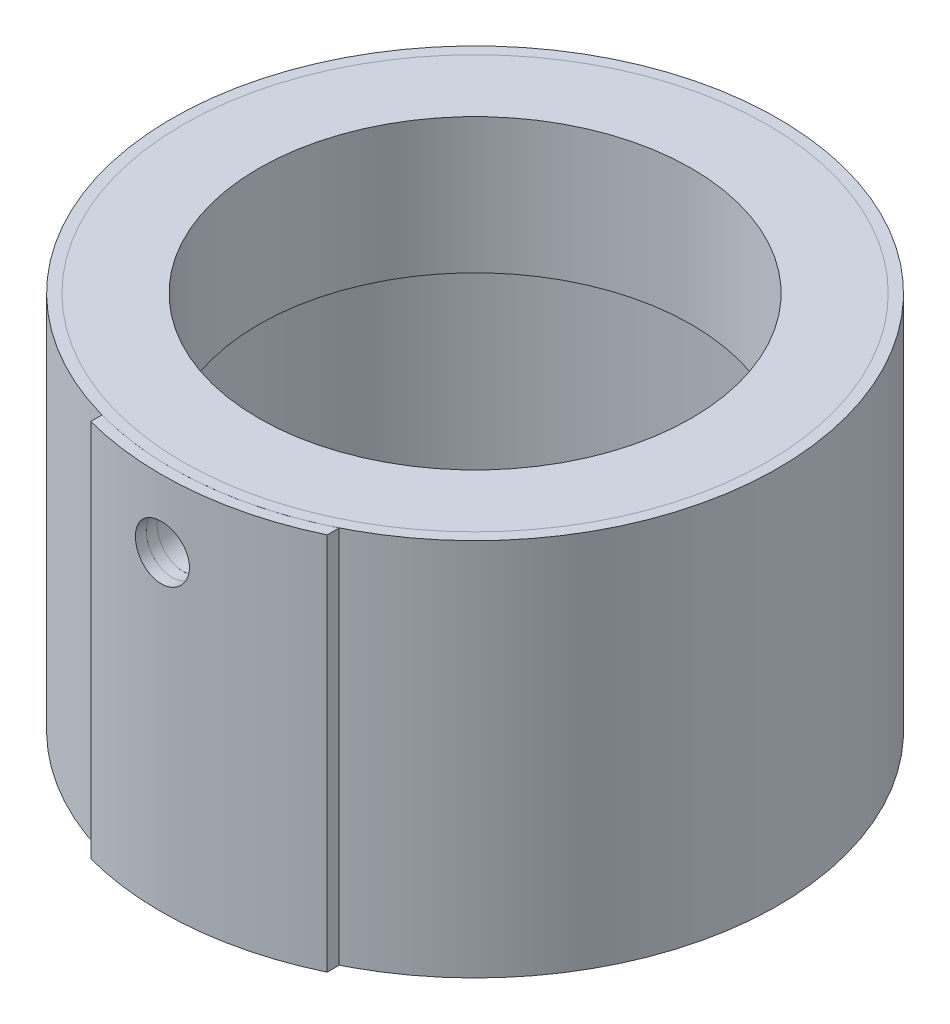
SolidWorks part; units mm, degrees
material "耐油橡胶Ⅰ- 2"
ref_plane "前视基准面" through (0, 0, 0) normal (0, 0, 1) x (1, 0, 0)
ref_plane "上视基准面" through (0, 0, 0) normal (0, 1, 0) x (1, 0, 0)
ref_plane "右视基准面" through (0, 0, 0) normal (1, 0, 0) x (0, 0, -1)
sketch "草图1" plane through (0, 0, 0) normal (0, 1, 0) x (1, 0, 0)
  circle A0 centre (0, 0) radius 40
  circle A1 centre (0, 0) radius 54
  dimension "D1" = 80
  dimension "D2" = 108
extrude "凸台-拉伸1" add sketch "草图1" along normal blind 25
sketch "草图2" plane through (0, 25, 0) normal (0, 1, 0) x (1, 0, 0)
  circle A0 centre (0, 0) radius 54 construction
  circle A1 centre (0, 0) radius 54
  circle A2 centre (0, 0) radius 56
  dimension "D1" = 2
extrude "凸台-拉伸2" add sketch "草图2" against normal blind 70 separate body
sketch "草图4" plane through (0, 25, 0) normal (0, 1, 0) x (1, 0, 0)
  line L0 (0, 0) -> (0, -58) construction
  line L1 (25, -50.1099) -> (25, -52.3355)
  line L2 (-15, -53.9537) -> (-15, -56.0268)
  line L3 (25, 0) -> (25, -58) construction
  line L4 (-15, 0) -> (-15, -58) construction
  circle A0 centre (0, 0) radius 56 construction
  arc A1 (-15, -53.9537) -> (25, -50.1099) centre (0, 0) ccw
  arc A2 (-15, -56.0268) -> (25, -52.3355) centre (0, 0) ccw
  circle A3 centre (0, 0) radius 58 construction
  circle A4 centre (0, 0) radius 56 construction
  dimension "D2" = 25
  dimension "D1" = 2
  dimension "D3" = 15
extrude "凸台-拉伸3" add sketch "草图4" against normal up to surface (70 mm away) separate body up to face at (0, -45, 54)
sketch "草图3" plane through (0, 0, 0) normal (0, 0, 1) x (1, 0, 0)
  line L0 (56, 25) -> (-56, 25) construction
  circle A0 centre (0, 12.5) radius 5
  dimension "D1" = 10
  dimension "D2" = 12.5
extrude "切除-拉伸1" cut sketch "草图3" along normal through all
